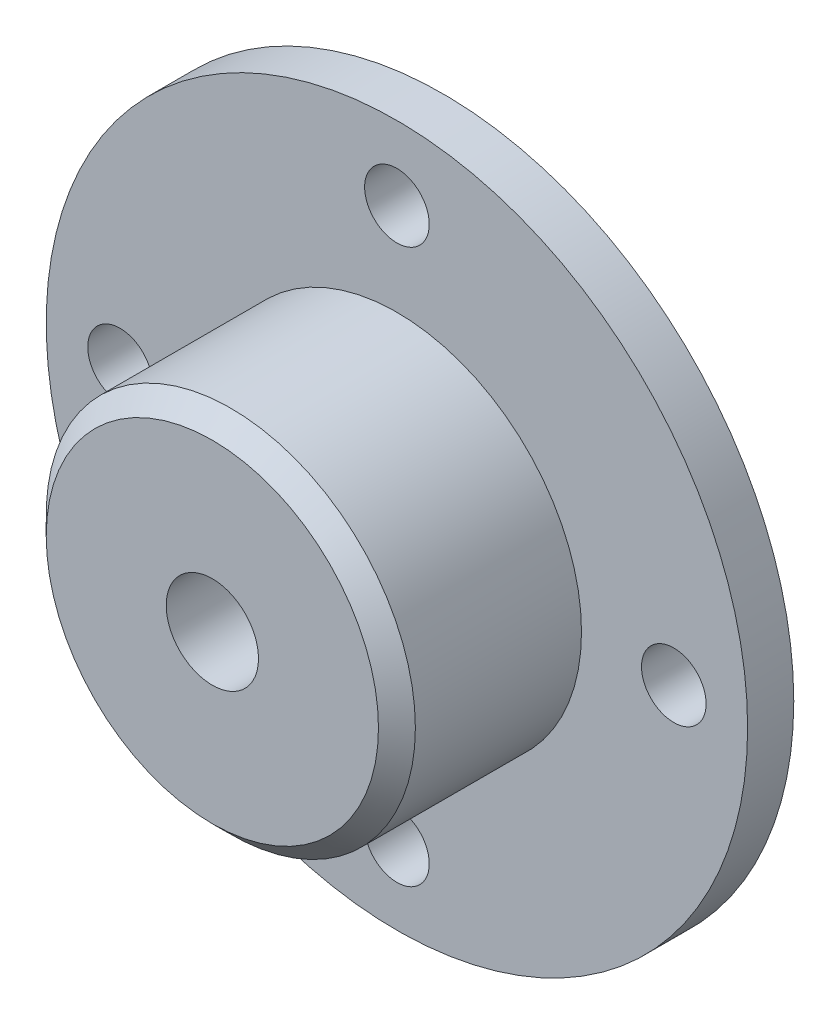
SolidWorks part; units mm, degrees
ref_plane "Front Plane" through (0, 0, 0) normal (0, 0, 1) x (1, 0, 0)
ref_plane "Top Plane" through (0, 0, 0) normal (0, 1, 0) x (1, 0, 0)
ref_plane "Right Plane" through (0, 0, 0) normal (1, 0, 0) x (0, 0, -1)
sketch "Sketch1" plane through (0, 0, 0) normal (0, 0, 1) x (1, 0, 0)
  circle A0 centre (0, 0) radius 19
  circle A1 centre (0, 0) radius 8.25
  dimension "D1" = 16.5
  dimension "D2" = 38
extrude "Boss-Extrude1" add sketch "Sketch1" along normal blind 2.5
sketch "Sketch2" plane through (0, 0, 2.5) normal (0, 0, 1) x (1, 0, 0)
  circle A0 centre (0, 0) radius 10
  dimension "D1" = 20
extrude "Boss-Extrude2" add sketch "Sketch2" along normal blind 10
sketch "Sketch3" plane through (0, 0, 2.5) normal (0, 0, 1) x (1, 0, 0)
  line L0 (0, 0) -> (50000, 0) construction
  line L1 (0, 0) -> (0, -50000) construction
  circle A0 centre (0, 0) radius 15 construction
  circle A1 centre (15, 0) radius 1.75
  circle A2 centre (0, 15) radius 1.75
  circle A3 centre (-15, 0) radius 1.75
  circle A4 centre (0, -15) radius 1.75
  dimension "D1" = 30
  dimension "D2" = 3.5
extrude "Cut-Extrude1" cut sketch "Sketch3" against normal blind 10
chamfer "Chamfer1" distance 1 angle 45 1 edges at (10, 0, 12.5)
hole_wizard "M6 Tapped Hole1" positions "Sketch6" profile "Sketch5" tap size "M6" standard "Gb" end condition through all
sketch "Sketch6" plane through (0, 0, 12.5) normal (0, 0, 1) x (1, 0, 0)
  point P0 (0, 0)
cosmetic thread "Cosmetic thread 1" parameters "D2"=6
sketch "Sketch5" plane through (0, 0, 12.5) normal (1, 0, 0) x (0, -1, 0)
  line L0 (0, 0) -> (0, 12.5)
  line L1 (0, 12.5) -> (2.5, 12.5)
  line L2 (2.5, 12.5) -> (2.5, 0)
  line L5 (2.5, 0) -> (0, 0)
  line L11 (0, -6.35) -> (0, 107.95) construction
  dimension "通孔螺纹孔钻头直径" = 5
  dimension "通孔螺纹孔钻头深度" = 12.5
